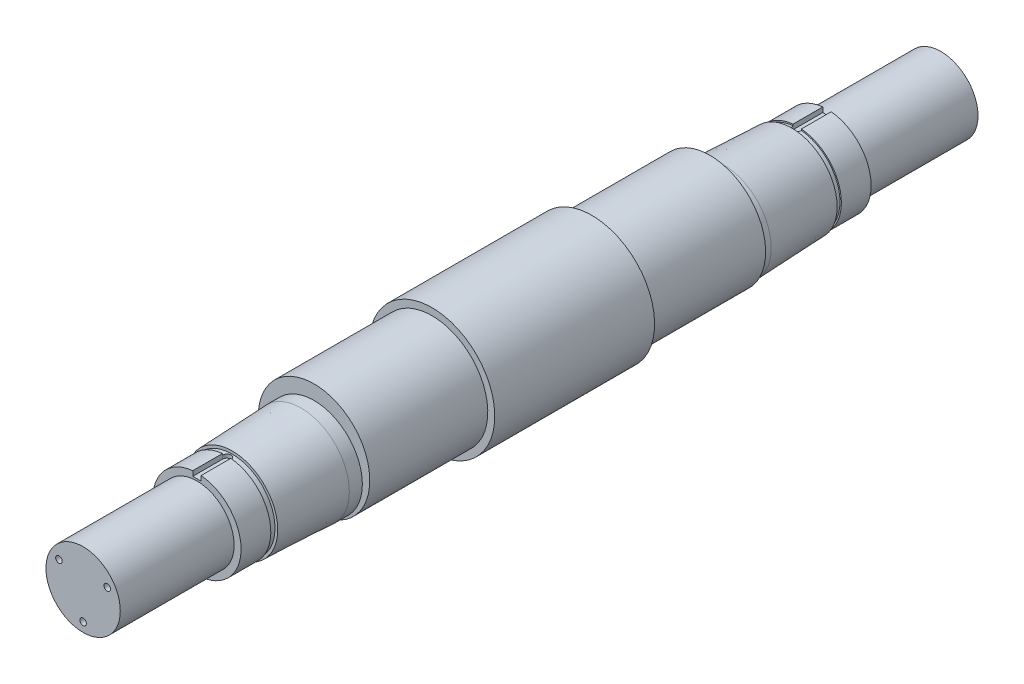
from build123d import *

# Parameters (mm, degrees)
CUT_EXTRUDE3_START = 95.1
CUT_EXTRUDE3_DEPTH = 26.1
CIRPATTERN1_COUNT  = 3


with BuildPart() as part:
    # Sketch2 → Revolve1 (revolve)
    with BuildSketch(Plane(origin=(0, 0, 0), x_dir=(0, 0, -1), z_dir=(1, 0, 0)), mode=Mode.PRIVATE) as revolve1_sk:
        Polygon((-172, 135), (172, 135), (172, 120), (426, 120), (426, 0), (0, 0), (-426, 0), (-426, 120), (-172, 120), align=None)
    revolve(revolve1_sk.sketch.rotate(Axis((0, 0, 564.378028921), (0, 0, -1)), 180), axis=Axis((0, 0, 564.378028921), (0, 0, -1)))

    # Sketch3 → Revolve2 (revolve)
    with BuildSketch(Plane(origin=(0, 0, 0), x_dir=(0, 0, -1), z_dir=(1, 0, 0)), mode=Mode.PRIVATE) as revolve2_sk:
        Polygon((426, -119), (426, -15), (923, -15), (923, -95), (678, -95), (678, -110), (614, -110), (614, -107), (602, -107), (602, -112.85), (454, -119), align=None)
    revolve2 = revolve(revolve2_sk.sketch.rotate(Axis((0, -15, 0), (0, 0, -1)), 270), axis=Axis((0, -15, 0), (0, 0, -1)))

    # Mirror1: Revolve2 across plane
    add(revolve2.mirror(Plane.XY))

    # Sketch5 → Cut-Extrude3 (cut)
    with BuildSketch(Plane(origin=(0, 0, 0), x_dir=(1, 0, 0), z_dir=(0, 1, 0)).offset(CUT_EXTRUDE3_START)):
        with BuildLine():
            Line((9, 742), (9, 614))
            ThreePointArc((9, 614), (0, 605), (-9, 614))
            Line((-9, 614), (-9, 742))
            ThreePointArc((-9, 742), (0, 751), (9, 742))
        make_face()
    cut_extrude3 = extrude(amount=-CUT_EXTRUDE3_DEPTH, mode=Mode.SUBTRACT)

    # Mirror2: Cut-Extrude3 across plane
    add(cut_extrude3.mirror(Plane.XY), mode=Mode.SUBTRACT)

    # Sketch7 → M16 Tapped Hole1 (revolve, cut)
    with BuildSketch(Plane(origin=(-51.961524227, 15, -923), x_dir=(0, 1, 0), z_dir=(1, 0, 0))):
        Polygon((0, 0), (0, 42.206024333), (7, 38), (7, 0), align=None)
    m16_tapped_hole1 = revolve(axis=Axis((-51.961524227, 15, -929.35), (0, 0, 1)), mode=Mode.SUBTRACT)

    # CirPattern1: M16 Tapped Hole1 ×3 about axis
    cirpattern1_axis = Axis((0, -15, 0), (0, 0, 1))
    for i in range(1, CIRPATTERN1_COUNT):
        add(m16_tapped_hole1.rotate(cirpattern1_axis, i * 360 / CIRPATTERN1_COUNT), mode=Mode.SUBTRACT)

    # Mirror3: M16 Tapped Hole1 across plane
    add(m16_tapped_hole1.mirror(Plane.XY), mode=Mode.SUBTRACT)

    # Mirror3 copy 1 sketch → Mirror3 copy 1 (revolve, cut)
    with BuildSketch(Plane(origin=(0, -75, 923), x_dir=(-0.8660254037844387, -0.4999999999999998, 0), z_dir=(-0.4999999999999998, 0.8660254037844387, 0))):
        Polygon((0, 0), (0, -42.206024333), (7, -38), (7, 0), align=None)
    revolve(axis=Axis((0, -75, 929.35), (0, 0, 1)), mode=Mode.SUBTRACT)

    # Mirror3 copy 2 sketch → Mirror3 copy 2 (revolve, cut)
    with BuildSketch(Plane(origin=(51.961524227, 15, 923), x_dir=(0.8660254037844384, -0.5000000000000004, 0), z_dir=(-0.5000000000000004, -0.8660254037844384, 0))):
        Polygon((0, 0), (0, -42.206024333), (7, -38), (7, 0), align=None)
    revolve(axis=Axis((51.961524227, 15, 929.35), (0, 0, 1)), mode=Mode.SUBTRACT)


solid = part.part
